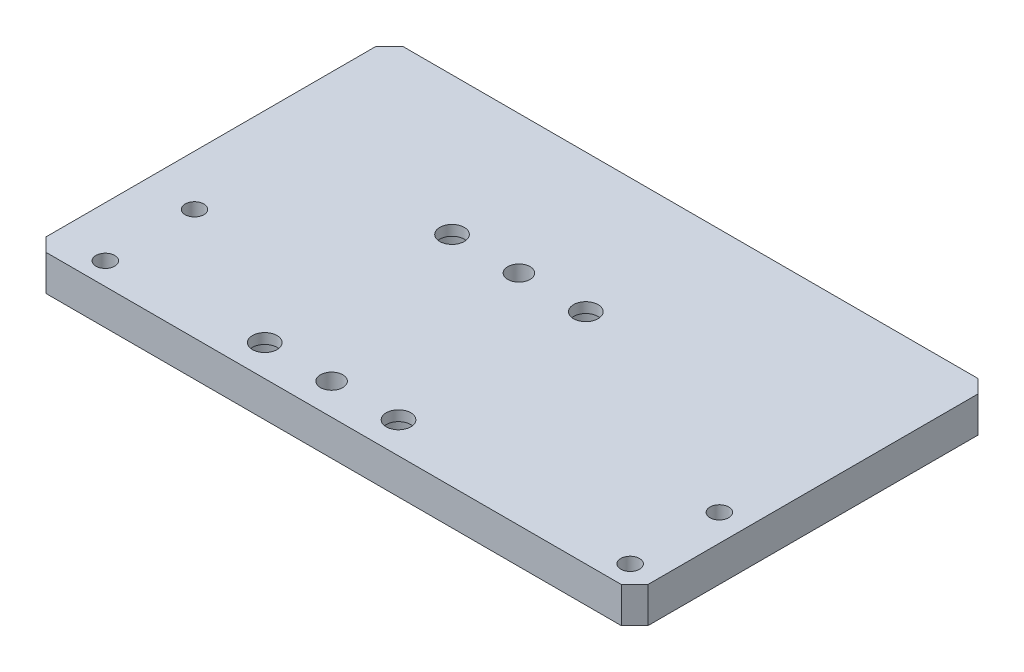
SolidWorks part; units mm, degrees
material "6061 合金"
ref_plane "Front Plane" through (0, 0, 0) normal (0, 0, 1) x (1, 0, 0)
ref_plane "Top Plane" through (0, 0, 0) normal (0, 1, 0) x (1, 0, 0)
ref_plane "Right Plane" through (0, 0, 0) normal (1, 0, 0) x (0, 0, -1)
sketch "Sketch1" plane through (0, 0, 0) normal (0, 1, 0) x (1, 0, 0)
  line L1 (0, 0) -> (135, 0)
  line L2 (0, 0) -> (0, 80)
  line L3 (0, 80) -> (135, 80)
  line L4 (135, 0) -> (135, 80)
  dimension "D1" = 80
  dimension "D2" = 135
extrude "Boss-Extrude1" add sketch "Sketch1" along normal blind 8
hole_wizard "CBORE for M5 Hexagon socket head cap screws1" positions "Sketch2" profile "Sketch3" counterbore size "M5" standard "GB" end condition through all
sketch "Sketch2" plane through (0, 0, 0) normal (0, -1, 0) x (-1, 0, 0)
  point P0 (-75.05, 49)
  point P3 (-45.05, 49)
  point P6 (-45.05, 7)
  point P9 (-75.05, 7)
sketch "Sketch3" plane through (75.05, 0, -49) normal (1, 0, 0) x (0, 0, -1)
  line L0 (0, 0) -> (0, 8)
  line L1 (0, 8) -> (2.75, 8)
  line L3 (2.75, 8) -> (2.75, 5.7)
  line L4 (2.75, 5.7) -> (5, 5.7)
  line L5 (5, 5.7) -> (5, 0)
  line L7 (5, 0) -> (0, 0)
  line L11 (0, -6.35) -> (0, 107.95) construction
  dimension "通孔孔直径" = 5.5
  dimension "通孔孔深度" = 8
  dimension "柱形沉头孔直径" = 10
  dimension "柱形沉头孔深度" = 5.7
hole_wizard "M5 Tapped Hole1" positions "Sketch4" profile "Sketch5" tap size "M5" standard "GB" end condition through all
sketch "Sketch4" plane through (0, 8, 0) normal (0, 1, 0) x (1, 0, 0)
  point P0 (129, 25)
  point P3 (129, 5)
  point P6 (11.3, 25)
  point P9 (11.3, 5)
sketch "Sketch5" plane through (129, 8, -25) normal (1, 0, 0) x (0, 0, 1)
  line L0 (0, 0) -> (0, 8)
  line L1 (0, 8) -> (2.1, 8)
  line L2 (2.1, 8) -> (2.1, 0)
  line L5 (2.1, 0) -> (0, 0)
  line L11 (0, -6.35) -> (0, 107.95) construction
  dimension "通孔螺纹孔钻头直径" = 4.2
  dimension "通孔螺纹孔钻头深度" = 8
cosmetic thread "Cosmetic Thread1"
cosmetic thread "Cosmetic Thread2"
cosmetic thread "Cosmetic Thread3"
cosmetic thread "Cosmetic Thread4"
chamfer "Chamfer1" distance 3 angle 45 4 edges at (0, 4, 0) (0, 4, -80) (135, 4, -80) (135, 4, 0)
hole_wizard "Ø5.0mm Dowel Hole1" positions "Sketch6" profile "Sketch7" hole size "Ø5.0" standard "GB" end condition through all
sketch "Sketch6" plane through (0, 0, 0) normal (0, -1, 0) x (-1, 0, 0)
  line L0 (-60.05, 48.5) -> (-60.05, 49.5) construction
  line L1 (-62.55, 49) -> (-57.55, 49) construction
  line L2 (-62.55, 48.5) -> (-62.55, 49.5) construction
  line L3 (-57.55, 49.5) -> (-57.55, 48.5) construction
  point P0 (-60.05, 7)
  point P3 (-60.05, 49)
sketch "Sketch7" plane through (60.05, 0, -7) normal (1, 0, 0) x (0, 0, -1)
  line L0 (0, 0) -> (0, 8)
  line L1 (0, 8) -> (2.5, 8)
  line L2 (2.5, 8) -> (2.5, 0)
  line L5 (2.5, 0) -> (0, 0)
  line L11 (0, -6.35) -> (0, 107.95) construction
  dimension "通孔孔直径" = 5
  dimension "通孔孔深度" = 8
